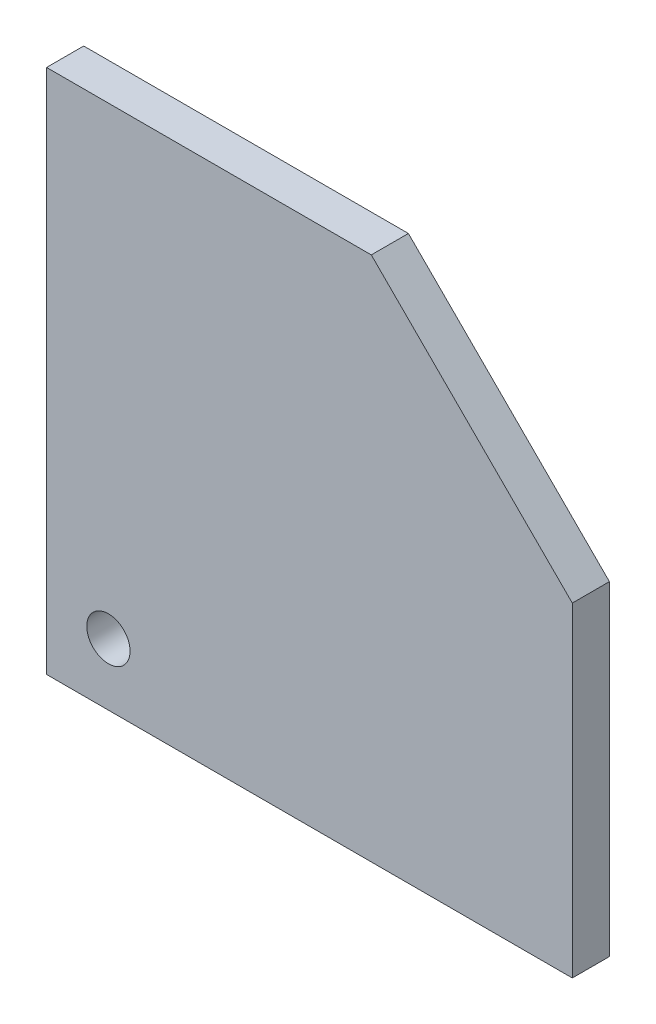
from build123d import *

# Parameters (mm, degrees)
SKETCH1_W              = 170
SKETCH1_H              = 170
EXTRUDE1_DEPTH         = 12
M16X2_0_TAPPED_HOLE1_D = 14
CHAMFER1_SIZE          = 65


with BuildPart() as part:
    # Sketch1 → Extrude1 (new body)
    with BuildSketch(Plane.XY):
        with Locations((85, 85)):
            Rectangle(SKETCH1_W, SKETCH1_H)
    extrude(amount=-EXTRUDE1_DEPTH)

    # M16x2.0 Tapped Hole1 (through all)
    with Locations(Plane.XY):
        with Locations((20, 20)):
            Hole(M16X2_0_TAPPED_HOLE1_D / 2)

    # Chamfer1
    chamfer1_edges = [part.edges().sort_by_distance(p)[0] for p in [
        (170, 170, -6),
    ]]
    chamfer(chamfer1_edges, length=CHAMFER1_SIZE)


solid = part.part
